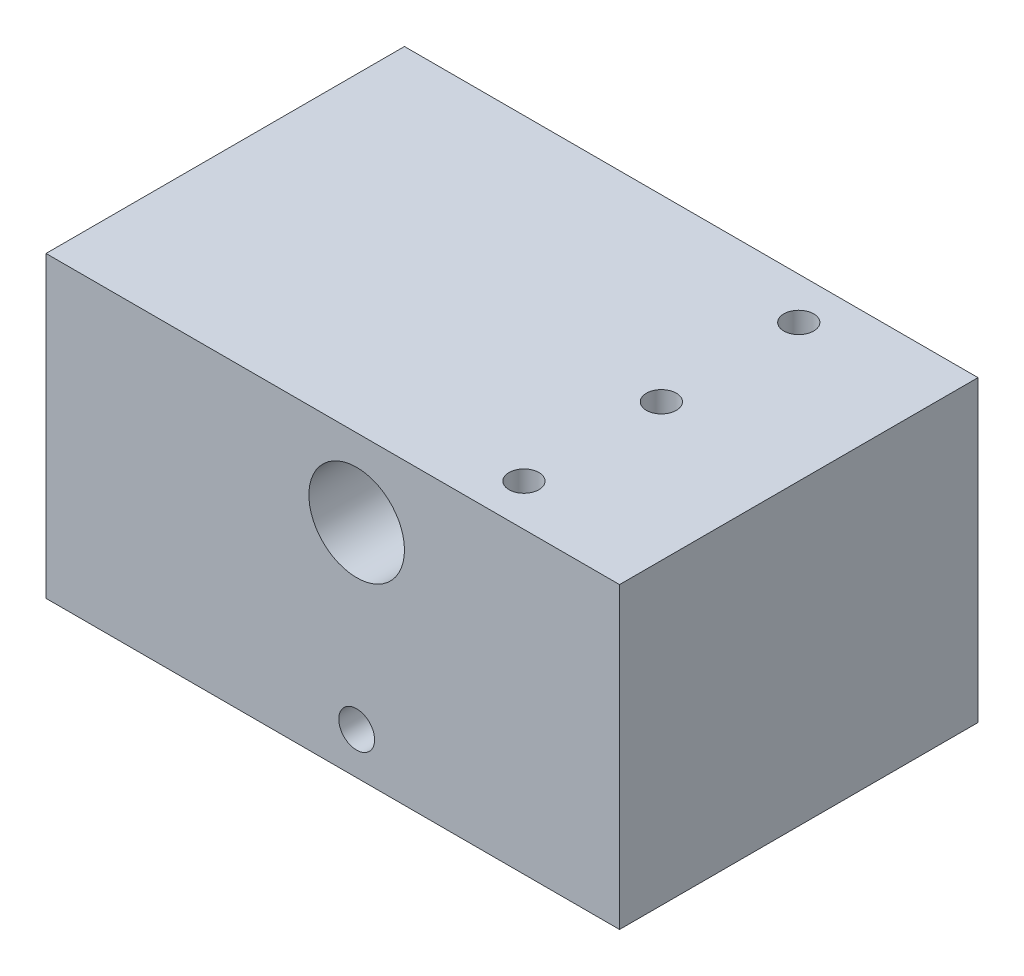
SolidWorks part; units mm, degrees
material "20#"
ref_plane "Front Plane" through (0, 0, 0) normal (0, 0, 1) x (1, 0, 0)
ref_plane "Top Plane" through (0, 0, 0) normal (0, 1, 0) x (1, 0, 0)
ref_plane "Right Plane" through (0, 0, 0) normal (1, 0, 0) x (0, 0, -1)
sketch "Sketch1" plane through (0, 0, 0) normal (0, 1, 0) x (1, 0, 0)
  line L1 (-24, 15) -> (24, 15)
  line L2 (-24, 15) -> (-24, -15)
  line L3 (-24, -15) -> (24, -15)
  line L4 (24, 15) -> (24, -15)
  line L5 (-24, 15) -> (24, -15) construction
  line L6 (-24, -15) -> (24, 15) construction
  point P0 (0, 0)
  dimension "D1" = 48
  dimension "D2" = 30
extrude "Boss-Extrude1" add sketch "Sketch1" along normal blind 25
sketch "Sketch3" plane through (0, 0, 15) normal (0, 0, 1) x (1, 0, 0)
  line L0 (24, 25) -> (-24, 25) construction
  circle A0 centre (2, 18.5) radius 4
  circle A1 centre (2, 3.5) radius 1.5
  dimension "D1" = 8
  dimension "D2" = 3
  dimension "D3" = 15
  dimension "D4" = 6.5
  dimension "D5" = 2
extrude "Cut-Extrude2" cut sketch "Sketch3" against normal up to next
sketch "Sketch4" plane through (0, 25, 0) normal (0, 1, 0) x (1, 0, 0)
  circle A0 centre (12.5, 11.5) radius 1
  circle A1 centre (12.5, 0) radius 1
  circle A2 centre (12.5, -11.5) radius 1
  dimension "D1" = 2
extrude "Cut-Extrude3" cut sketch "Sketch4" against normal blind 2
hole_wizard "M3 Tapped Hole1" positions "Sketch5" profile "Sketch6" tap size "M3" standard "GB"
sketch "Sketch5" plane through (0, 25, 0) normal (0, 1, 0) x (1, 0, 0)
  point P0 (12.5, 11.5)
  point P3 (12.5, 0)
  point P6 (12.5, -11.5)
sketch "Sketch6" plane through (12.5, 25, -11.5) normal (1, 0, 0) x (0, 0, 1)
  line L0 (0, 0) -> (0, 8.2511)
  line L1 (0, 8.2511) -> (1.25, 7.5)
  line L2 (1.25, 7.5) -> (1.25, 0)
  line L5 (1.25, 0) -> (0, 0)
  line L10 (0, 8.2511) -> (-1.25, 7.5) construction
  line L11 (0, -6.35) -> (0, 107.95) construction
  dimension "螺纹孔钻头直径" = 2.5
  dimension "螺纹孔钻头深度" = 7.5
  dimension "导头角度" = 118
cosmetic thread "HoleThreadLine1" parameters "D1"=6, "D2"=3
cosmetic thread "HoleThreadLine2" parameters "D1"=6, "D2"=3
cosmetic thread "HoleThreadLine3" parameters "D1"=6, "D2"=3
